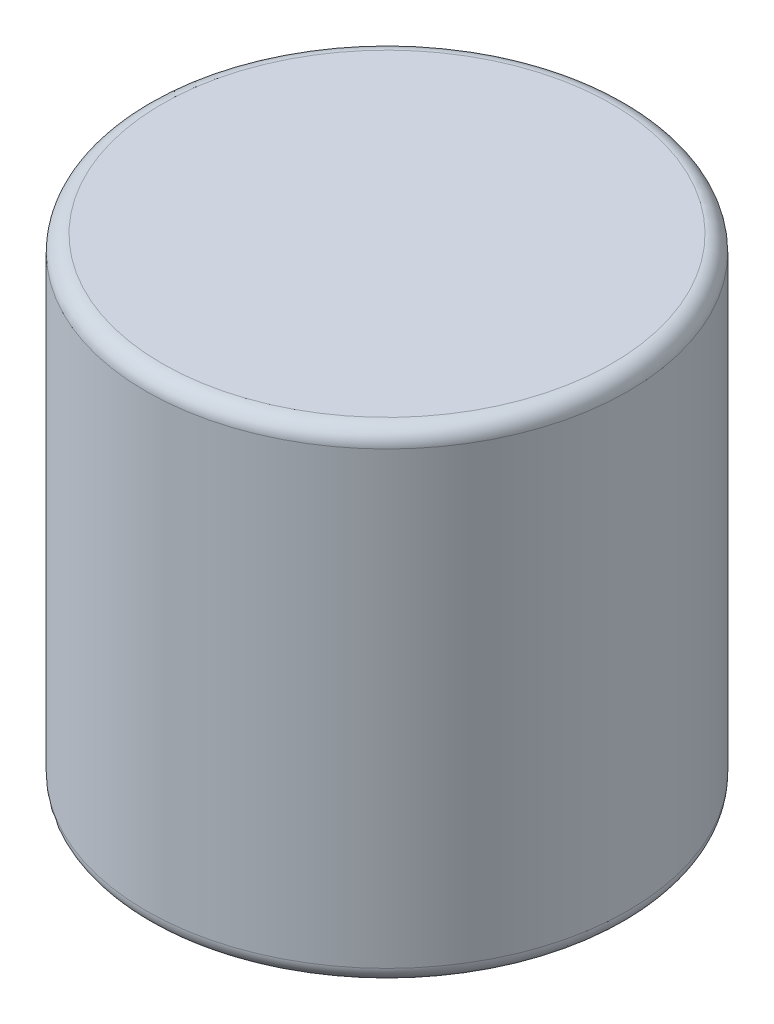
from build123d import *

# Parameters (mm, degrees)
FILLET1_R = 10


with BuildPart() as part:
    # Sketch1 → Revolve1 (revolve)
    with BuildSketch(Plane.XY, mode=Mode.PRIVATE) as revolve1_sk:
        Polygon((0, 0), (0, 370), (150, 370), (150, 70), (20, 70), (20, 30), (15, 30), (15, 0), align=None)
    revolve(revolve1_sk.sketch.rotate(Axis((0, 0, 0), (0, 1, 0)), 90), axis=Axis((0, 0, 0), (0, 1, 0)))

    # Fillet1
    fillet1_edges = [part.edges().sort_by_distance(p)[0] for p in [
        (0, 70, 150),
        (0, 370, 150),
    ]]
    fillet(fillet1_edges, radius=FILLET1_R)


solid = part.part
